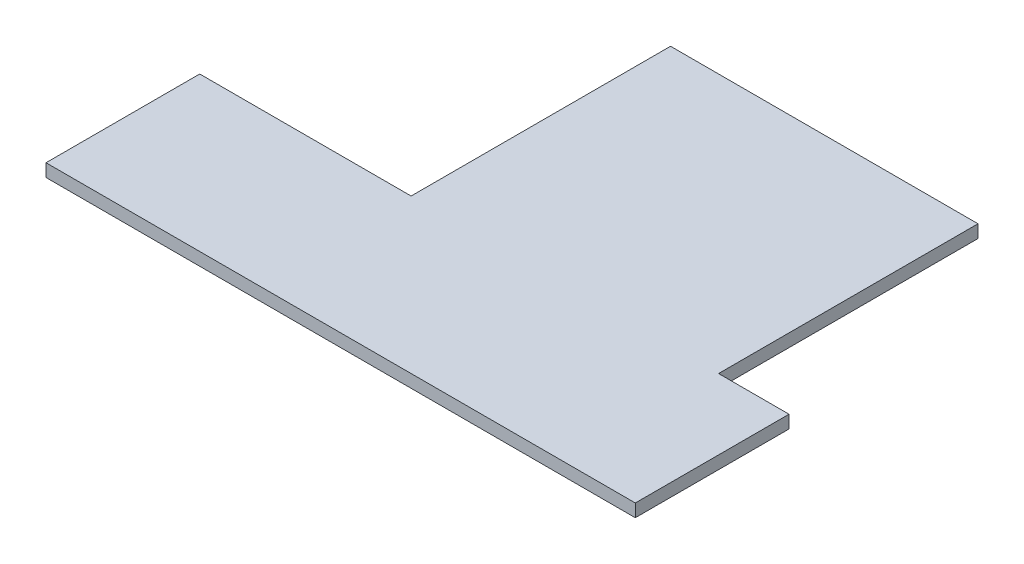
SolidWorks part; units mm, degrees
ref_plane "Front Plane" through (0, 0, 0) normal (0, 0, 1) x (1, 0, 0)
ref_plane "Top Plane" through (0, 0, 0) normal (0, 1, 0) x (1, 0, 0)
ref_plane "Right Plane" through (0, 0, 0) normal (1, 0, 0) x (0, 0, -1)
sketch "Sketch1" plane through (0, 0, 0) normal (0, 1, 0) x (1, 0, 0)
  line L0 (-330, -655) -> (590, -655)
  line L1 (590, -655) -> (590, -415)
  line L2 (590, -415) -> (480, -415)
  line L3 (0, -415) -> (-330, -415)
  line L4 (-330, -415) -> (-330, -655)
  line L5 (0, -415) -> (0, -10)
  line L7 (480, -10) -> (480, -415)
  line L9 (480, -10) -> (0, -10)
  dimension "D1" = 330
  dimension "D2" = 110
  dimension "D3" = 240
  dimension "D4" = 920
  dimension "D5" = 415
  dimension "D6" = 110
extrude "Boss-Extrude1" add sketch "Sketch1" along normal blind 20
